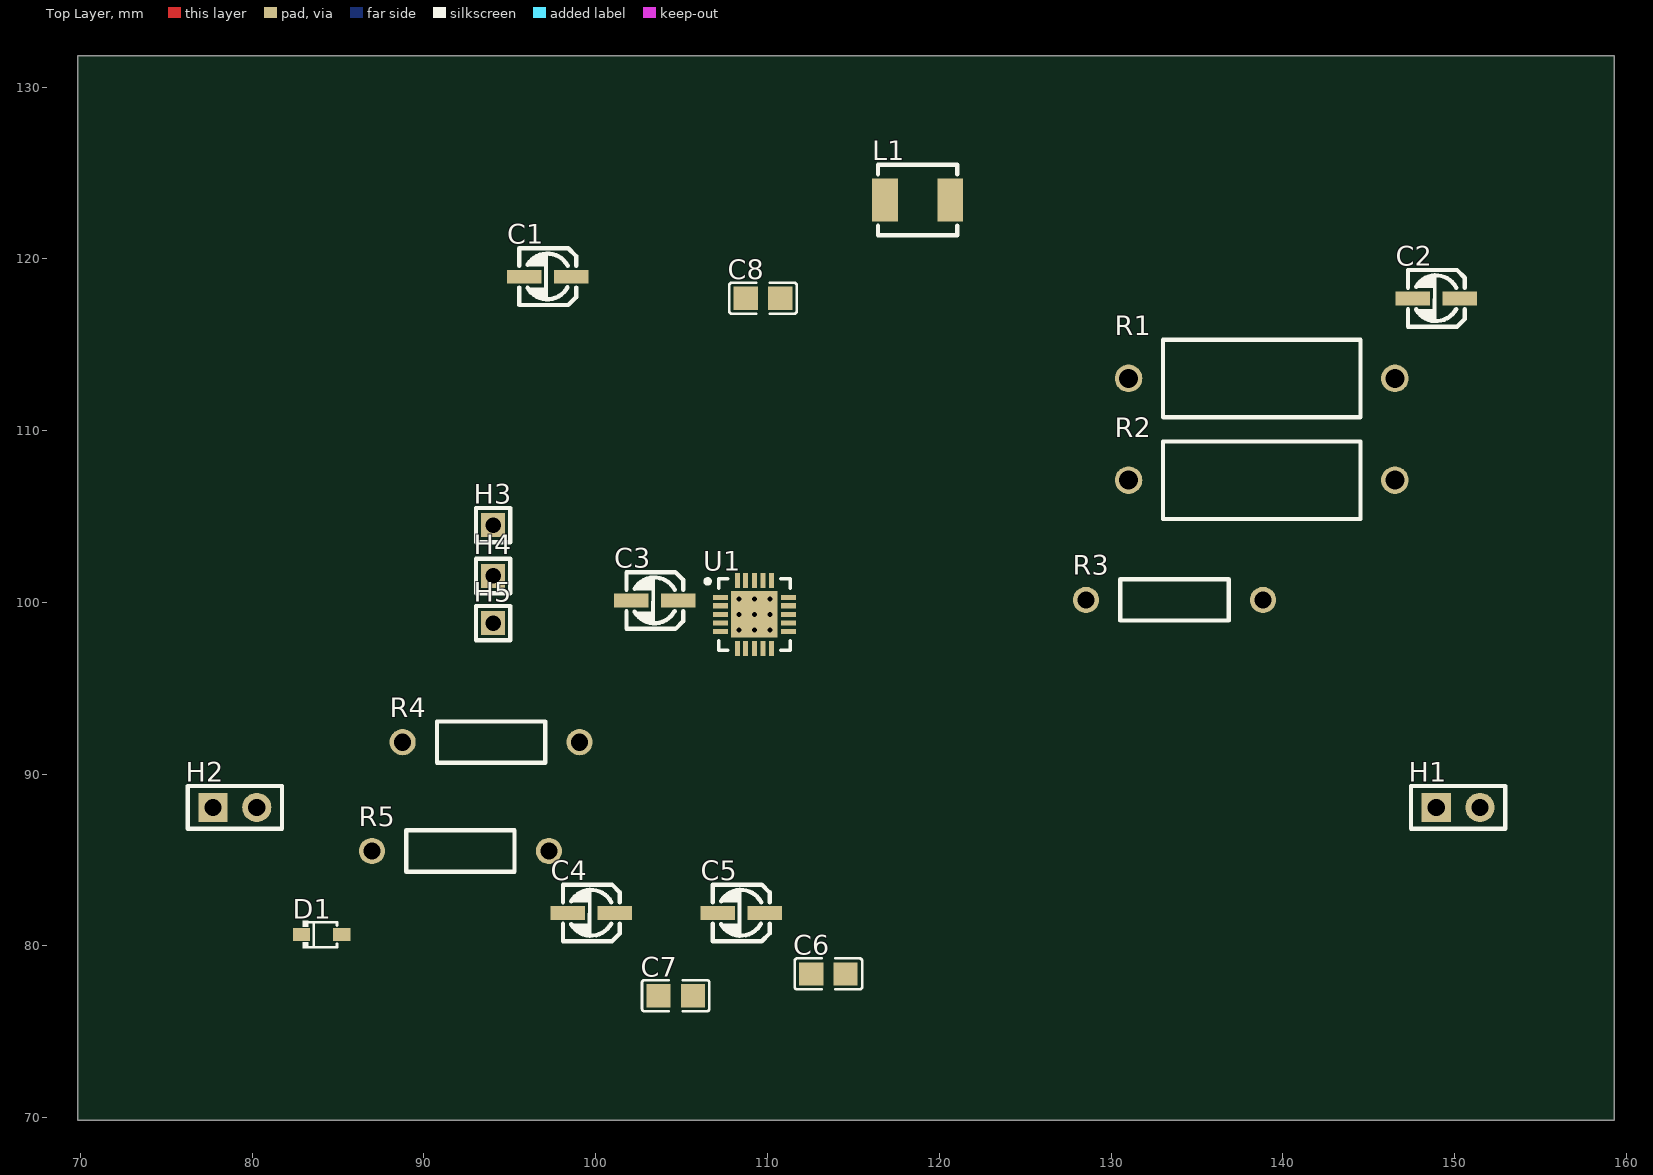
[diagram p0: Top Layer view]
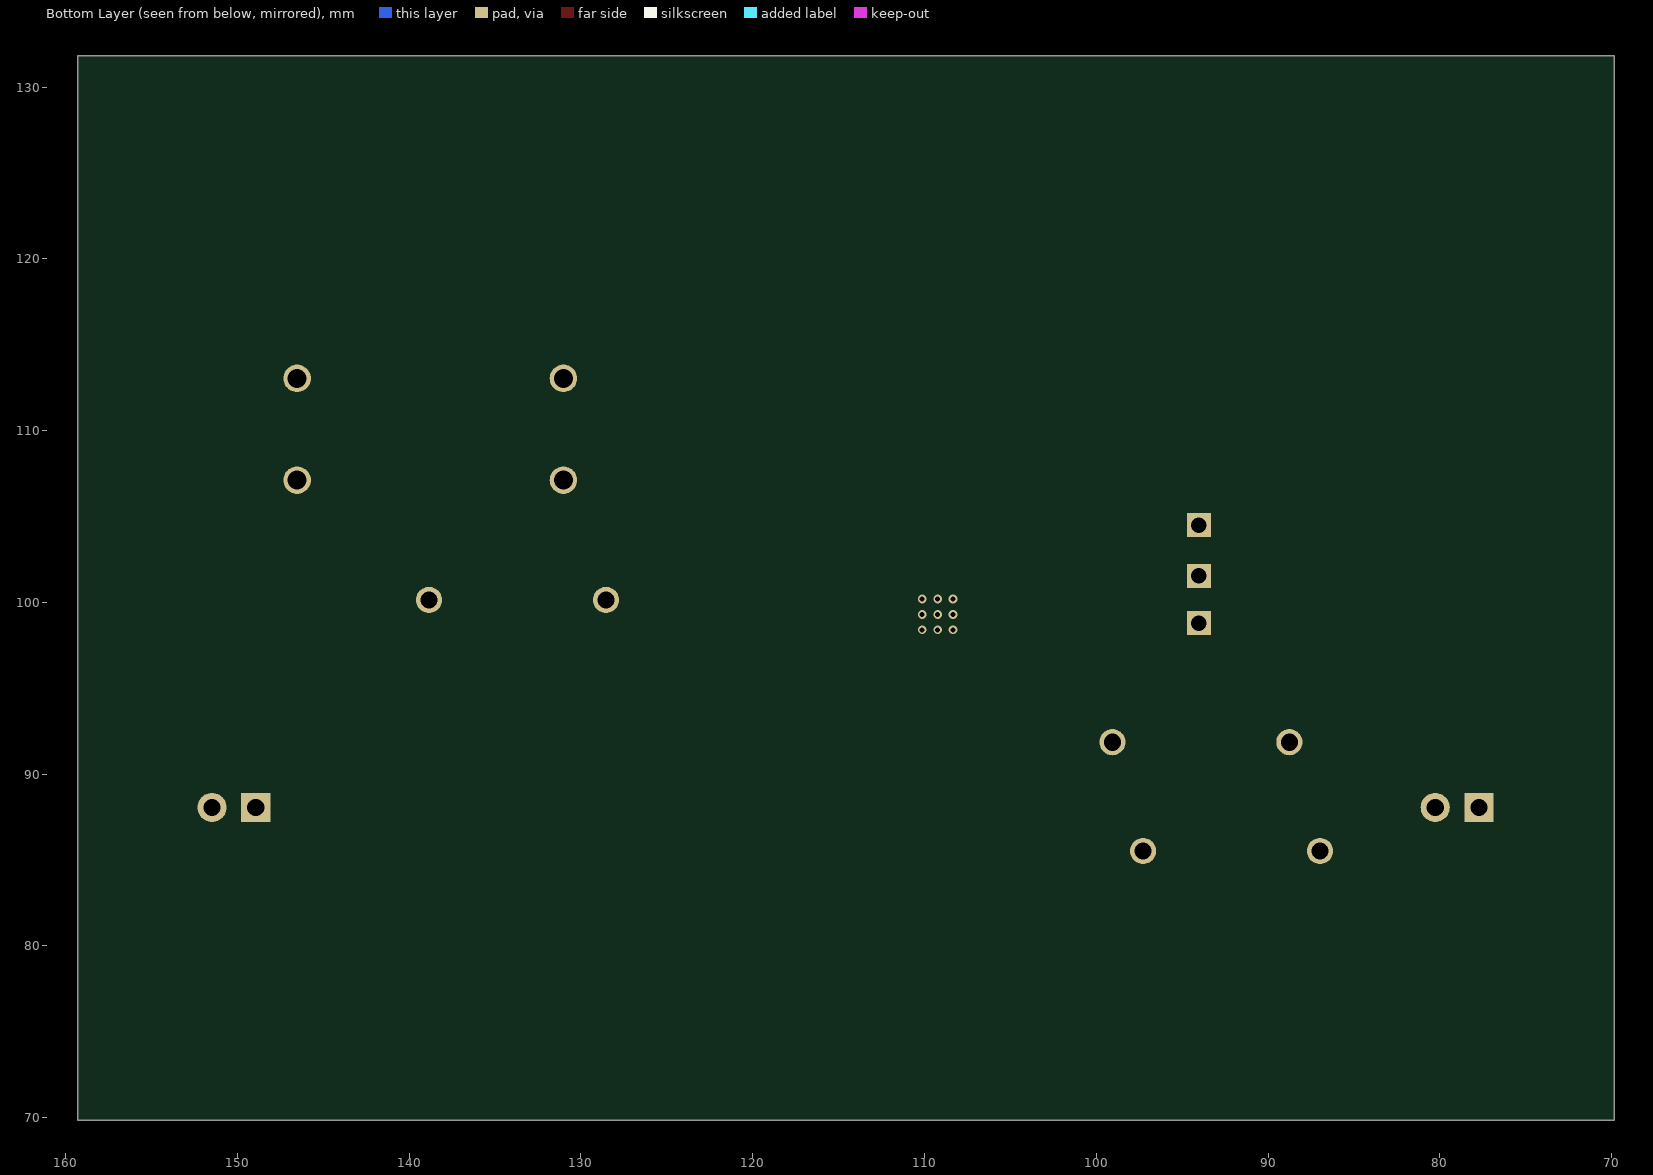
[diagram p1: Bottom Layer view, seen from below]
# Altium PCB MISC51337.pcbdoc
Units mm, origin at the board's own origin, x right, y up, seen from the top; angles counter-clockwise.
Board outline 89.44 x 61.97 mm, 2 copper layers (Top Layer, Bottom Layer), stack 0.07 mm thick; 21 components, 16 nets, 58 pads, 9 vias.

## Layer stack, top to bottom
Top Solder Mask Layer: solder mask 0.01, Dk 3.3
Top Layer: signal copper 0.035
Bottom Layer: signal copper 0.035
Bottom Solder Mask Layer: solder mask 0.01, Dk 3.3

## Board outline
159.293,69.85 69.85,69.85 69.85,131.82 159.293,131.82

## Design rules (kind name [scope] priority, off if disabled: settings)
BoardOutlineClearance Plane_innerPlane_1 [All] p2 off: genericclearance=0.102 ignorepadtopadclearanceinfootprint=FALSE except(0: Arc-SplitContinuation Track-SplitContinuation SMDPad-SplitContinuation THPad-SplitContinuation Via-SplitContinuation Fill-SplitContinuation Region-SplitContinuation Poly-SplitContinuation Text-SplitContinuation Hole-SplitContinuation; 0.152: Arc-CutoutEdge Track-CutoutEdge SMDPad-CutoutEdge THPad-CutoutEdge Via-CutoutEdge Text-CutoutEdge; 0.175: Hole-OutlineEdge Hole-CutoutEdge; 0.254: Poly-OutlineEdge Poly-CutoutEdge; 0.3: Arc-OutlineEdge Track-OutlineEdge SMDPad-OutlineEdge THPad-OutlineEdge Via-OutlineEdge Fill-OutlineEdge Region-OutlineEdge Text-OutlineEdge Fill-CutoutEdge Region-CutoutEdge)
BoardOutlineClearance Copper_copperRegion_1 [All] p4 off: genericclearance=0.102 ignorepadtopadclearanceinfootprint=FALSE except(0: Arc-SplitContinuation Track-SplitContinuation SMDPad-SplitContinuation THPad-SplitContinuation Via-SplitContinuation Fill-SplitContinuation Region-SplitContinuation Poly-SplitContinuation Text-SplitContinuation Hole-SplitContinuation; 0.152: Arc-CutoutEdge Track-CutoutEdge SMDPad-CutoutEdge THPad-CutoutEdge Via-CutoutEdge Text-CutoutEdge; 0.175: Hole-OutlineEdge Hole-CutoutEdge; 0.254: Poly-OutlineEdge Poly-CutoutEdge; 0.3: Arc-OutlineEdge Track-OutlineEdge SMDPad-OutlineEdge THPad-OutlineEdge Via-OutlineEdge Fill-OutlineEdge Region-OutlineEdge Text-OutlineEdge Fill-CutoutEdge Region-CutoutEdge)
BoardOutlineClearance copperThickness1oz_1 [All] p6: genericclearance=0.102 ignorepadtopadclearanceinfootprint=FALSE except(0: Arc-SplitContinuation Track-SplitContinuation SMDPad-SplitContinuation THPad-SplitContinuation Via-SplitContinuation Fill-SplitContinuation Region-SplitContinuation Poly-SplitContinuation Text-SplitContinuation Hole-SplitContinuation; 0.152: Arc-CutoutEdge Track-CutoutEdge SMDPad-CutoutEdge THPad-CutoutEdge Via-CutoutEdge Text-CutoutEdge; 0.175: Hole-OutlineEdge Hole-CutoutEdge; 0.254: Poly-OutlineEdge Poly-CutoutEdge; 0.3: Arc-OutlineEdge Track-OutlineEdge SMDPad-OutlineEdge THPad-OutlineEdge Via-OutlineEdge Fill-OutlineEdge Region-OutlineEdge Text-OutlineEdge Fill-CutoutEdge Region-CutoutEdge)
Clearance Plane_innerPlane [All] p1 off: gap=0.102 ignorepadtopadclearanceinfootprint=FALSE except(0.152: SMDPad-Track SMDPad-SMDPad THPad-Track SMDPad-THPad THPad-THPad Track-Via SMDPad-Via THPad-Via Via-Via Fill-SMDPad Region-SMDPad Fill-THPad Region-THPad Fill-Via Region-Via Fill-Fill Fill-Region Region-Region Arc-Track Arc-SMDPad Arc-THPad Arc-Via Fill-Arc Region-Arc Arc-Arc Text-Track SMDPad-Text Text-THPad Text-Via Fill-Text Region-Text Arc-Text Text-Text; 0.175: Hole-Track Hole-SMDPad Hole-THPad Hole-Via Fill-Hole Region-Hole Hole-Arc Hole-Text; 0.254: Poly-Track Poly-SMDPad Poly-THPad Poly-Via Poly-Fill Poly-Region Poly-Poly Poly-Arc Poly-Text Poly-Hole; 0.3: Fill-Track Region-Track)
Clearance Copper_copperRegion [All] p3 off: gap=0.102 ignorepadtopadclearanceinfootprint=FALSE except(0.152: SMDPad-Track SMDPad-SMDPad THPad-Track SMDPad-THPad THPad-THPad Track-Via SMDPad-Via THPad-Via Via-Via Fill-SMDPad Region-SMDPad Fill-THPad Region-THPad Fill-Via Region-Via Fill-Fill Fill-Region Region-Region Arc-Track Arc-SMDPad Arc-THPad Arc-Via Fill-Arc Region-Arc Arc-Arc Text-Track SMDPad-Text Text-THPad Text-Via Fill-Text Region-Text Arc-Text Text-Text; 0.175: Hole-Track Hole-SMDPad Hole-THPad Hole-Via Fill-Hole Region-Hole Hole-Arc Hole-Text; 0.254: Poly-Track Poly-SMDPad Poly-THPad Poly-Via Poly-Fill Poly-Region Poly-Poly Poly-Arc Poly-Text Poly-Hole; 0.3: Fill-Track Region-Track)
Clearance copperThickness1oz [All] p5: gap=0.102 ignorepadtopadclearanceinfootprint=FALSE except(0.152: SMDPad-Track SMDPad-SMDPad THPad-Track SMDPad-THPad THPad-THPad Track-Via SMDPad-Via THPad-Via Via-Via Fill-SMDPad Region-SMDPad Fill-THPad Region-THPad Fill-Via Region-Via Fill-Fill Fill-Region Region-Region Arc-Track Arc-SMDPad Arc-THPad Arc-Via Fill-Arc Region-Arc Arc-Arc Text-Track SMDPad-Text Text-THPad Text-Via Fill-Text Region-Text Arc-Text Text-Text; 0.175: Hole-Track Hole-SMDPad Hole-THPad Hole-Via Fill-Hole Region-Hole Hole-Arc Hole-Text; 0.254: Poly-Track Poly-SMDPad Poly-THPad Poly-Via Poly-Fill Poly-Region Poly-Poly Poly-Arc Poly-Text Poly-Hole; 0.3: Fill-Track Region-Track)
DiffPairsRouting differentialPair [All] p1: maxlimit=0.152 minlimit=0.127 mostfreqgap=0.152 toplayer_minwidth=0.127 toplayer_prefwidth=2.54 toplayer_maxwidth=2.54 toplayer_mingap=0.127 toplayer_prefgap=0.152 toplayer_maxgap=0.152 bottomlayer_minwidth=0.127 bottomlayer_prefwidth=2.54 bottomlayer_maxwidth=2.54 bottomlayer_mingap=0.127 bottomlayer_prefgap=0.152 bottomlayer_maxgap=0.152 maxuncoupledlength=0.254
HoleToHoleClearance otherClearance [All] p1: gap=0.3 allowstackedmicrovias=TRUE
Length netLength [All] p1: minlimit=0 maxlimit=0
PasteMaskExpansion pasteMaskExpansion [All] p1: expansion=0
PlaneConnect innerPlane [All] p1: planeconnectstyle=Relief reliefexpansion=0.508 reliefentries=4 reliefconductorwidth=0.254 reliefairgap=0.254
PolygonConnect copperRegion [All] p1: connectstyle=Relief reliefconductorwidth=0.254 reliefentries=4 polygonreliefangle="90 Angle" airgapwidth=0.254 via.connectstyle=Relief via.reliefconductorwidth=0.254 via.reliefentries=4 via.polygonreliefangle="90 Angle" via.airgapwidth=0.254
RoutingVias viaSize [All] p1: holewidth=0.61 width=0.305 viastyle="Through Hole" minholewidth=0.5 minwidth=0.3 maxholewidth=10 maxwidth=6.299
SolderMaskExpansion solderMaskExpansion [IsVia] p1: expansion=-25.4 istentingtop=TRUE
SolderMaskExpansion solderMaskExpansion [All] p2: expansion=0.051 istentingtop=FALSE
Width copperThickness1oz_2 [All] p1: maxlimit=2.54 minlimit=0.127 preferedwidth=0.254

## Components (designator, comment, footprint, x,y, rotation, side; value= is the part's Value field where it differs from the comment)
C1 "0.1uF" C_Ele_SMD_3x5.4mm 97.204,118.974 r0 top
C2 "100nF/250V" C_Ele_SMD_3x5.4mm 148.933,117.704 r0 top
C3 "0.1u" C_Ele_SMD_3x5.4mm 103.438,100.117 r0 top
C4 "10nF" C_Ele_SMD_3x5.4mm 99.744,81.928 r0 top
C5 "10nF" C_Ele_SMD_3x5.4mm 108.468,81.928 r0 top
C6 "100nF" C0805 113.548,78.374 r0 top
C7 "100nF" C0805 104.658,77.104 r0 top
C8 "10u" C0805 109.738,117.704 r0 top
D1 "BAT165E6327" SOD-323_L1.8-W1.3-LS2.5-RD 84.039,80.658 r0 top
H1 "" HDR-TH_2P-P2.54-V-F 150.203,88.064 r0 top
H2 "" HDR-TH_2P-P2.54-V-F 79,88.064 r0 top
H3 "" HDR-TH_1P-V-M_XKB_X4611WV-01I-C28D40 94.029,104.496 r0 top
H4 "" HDR-TH_1P-V-M_XKB_X4611WV-01I-C28D40 94.029,101.542 r0 top
H5 "" HDR-TH_1P-V-M_XKB_X4611WV-01I-C28D40 94.029,98.788 r0 top
L1 "4.7uH" IND-SMD_L4.6-W4.1-A 118.737,123.42 r0 top
R1 "1.72M" Res_1W 138.773,113.04 r0 top
R2 "15k" Res_1W 138.773,107.113 r0 top
R3 "18k" Res_1/4W 133.693,100.145 r0 top
R4 "1k" Res_1/4W 93.913,91.862 r0 top
R5 "1k" Res_1/4W 92.124,85.524 r0 top
U1 "DRV2700" TI-RGP20-2700X2700TP_V 109.241,99.296 r0 top

## Footprints (in the part's own frame and the unit in brackets; to place one, negate y for a bottom-side part, rotate by r counter-clockwise, add the part's x,y. Pads: shape width x height; smd on the part's side, far side on the other; paste and mask are expansions set on the pad)
C0805 [mm]
  rect 1.41x1.35 smd paste-100 mask+0.051: 1(-1,0) 2(1,0)
  silkscreen extent -1.96,-0.9 1.96,0.9
C_Ele_SMD_3x5.4mm [mil]
  rect 78.7x31.5 smd paste+0 mask+2: 1(54.1,-0.55) 2(-53.7,-0.55)
  silkscreen extent -65,-65 65,65
HDR-TH_1P-V-M_XKB_X4611WV-01I-C28D40 [mm]
  rect 1.4x1.4 hole 0.9: 1(0,0)
  silkscreen extent -1,-1 1,1
HDR-TH_2P-P2.54-V-F [mm]
  rect 1.7x1.7 hole 1: 1(-1.27,0)
  round 1.7 hole 1: 2(1.27,0)
  silkscreen extent -2.74,-1.25 2.74,1.25
IND-SMD_L4.6-W4.1-A [mm]
  rect 1.5x2.5 smd: 1(-1.9,0) 2(1.9,0)
  silkscreen extent -2.3,-2.05 2.3,2.05
Res_1/4W [mm]
  round 1.524 hole 1 paste+0 mask+0.051: 1(-5.15,0) 2(5.15,0)
  silkscreen extent -3.15,-1.2 3.15,1.2
Res_1W [mm]
  round 1.6 hole 1.1 paste+0 mask+0.051: 1(-7.75,0) 2(7.75,0)
  silkscreen extent -5.75,-2.26 5.75,2.25
SOD-323_L1.8-W1.3-LS2.5-RD [mm]
  rect 1x0.75 smd: 1(-1.173,0) 2(1.173,0)
  silkscreen extent -1.08,-0.8 0.9,0.8
TI-RGP20-2700X2700TP_V [mil]
  rect 34.5x11.5 smd paste+0 mask+4: 1(-78,39) 2(-78,20) 3(-78,0) 4(-78,-20) 5(-78,-39) 11(78,-39) 12(78,-20) 13(78,0) 14(78,20) 15(78,39)
  rect 11.5x34.5 smd paste+0 mask+4: 6(-39,-78) 7(-20,-78) 8(0,-78) 9(20,-78) 10(39,-78) 16(39,78) 17(20,78) 18(0,78) 19(-20,78) 20(-39,78)
  rect 106.5x106.5 smd paste+0 mask+4: 21(0,0)
  silkscreen extent -112,-82 82,82

## Via types
v1: diameter 0.5, hole 0.3, Top Layer to Bottom Layer, 9 vias

## Nets (pads, with @x,y where several pads share a name; then routed paths per layer and width w, separated by ;. In a path a pad name is that pad's centre, name@x,y a point inside that pad or via, vN(x,y) a via of type N, cw(c..) or ccw(c..) an arc to the next point about the centre after c; other vN are vias at no path point)
$1N1: H1.1 U1.13
$1N2: H1.2 U1.14
$1N6: L1.2 U1.8
$1N7: C2.1 R1.2 U1.10 U1.12
$1N8: R1.1 R2.2 U1.3
$1N11: H3.1 U1.20
$1N12: H4.1 U1.18
$1N13: H5.1 U1.19
$1N14: C3.1 U1.1
$1N16: R3.2 U1.15
$1N18: C4.1 C7.2 R4.2 U1.17
$1N19: C5.1 C6.2 R5.2 U1.16
$1N22: D1.1 H2.1 R5.1
$1N23: H2.2 R4.1
GND: C1.2 C2.2 C3.2 C4.2 C5.2 C6.1 C7.1 C8.1 D1.2 R2.1 R3.1 U1.4 U1.5 U1.6 U1.21
  other v1: 108.341,98.397 109.241,98.397 110.14,98.397 108.341,99.296 109.241,99.296 110.14,99.296 108.341,100.195 109.241,100.195 110.14,100.195
VCC: C1.1 C8.2 L1.1 U1.2
pads on no net: U1.7 U1.9 U1.11